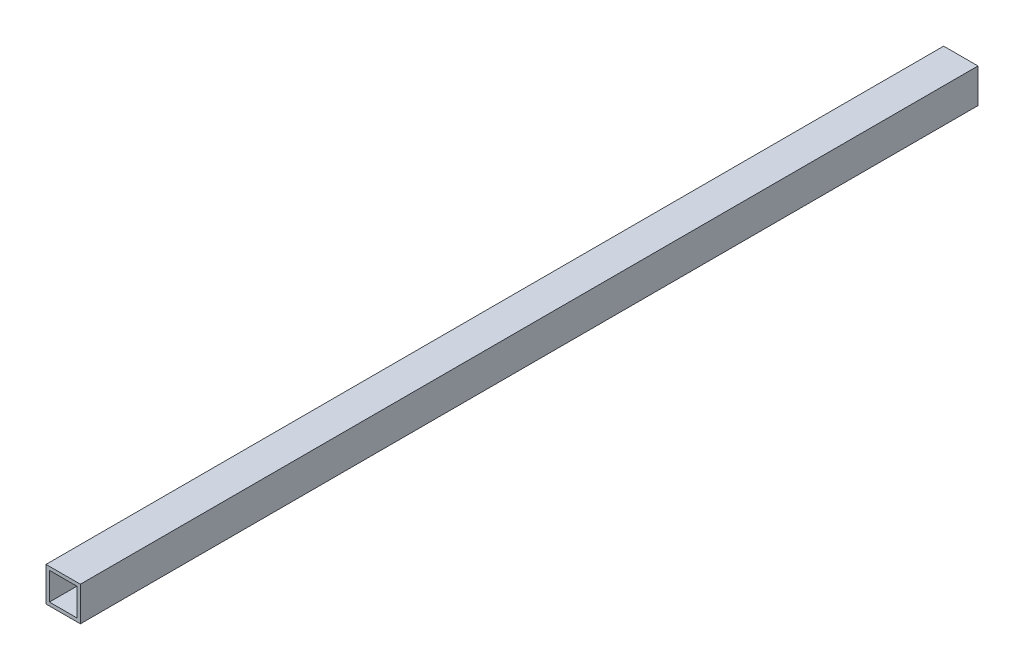
SolidWorks part; units mm, degrees
ref_plane "Front Plane" through (0, 0, 0) normal (0, 0, 1) x (1, 0, 0)
ref_plane "Top Plane" through (0, 0, 0) normal (0, 1, 0) x (1, 0, 0)
ref_plane "Right Plane" through (0, 0, 0) normal (1, 0, 0) x (0, 0, -1)
other "Configuration Table"
sketch "Sketch1" plane through (0, 0, 0) normal (0, 0, 1) x (1, 0, 0)
  line L0 (-16.1154, 15.8464) -> (13.8846, 15.8464)
  line L1 (13.8846, 15.8464) -> (13.8846, -14.1536)
  line L2 (13.8846, -14.1536) -> (-16.1154, -14.1536)
  line L3 (-16.1154, -14.1536) -> (-16.1154, 15.8464)
  line L4 (-13.1154, 12.8464) -> (10.8846, 12.8464)
  line L5 (10.8846, 12.8464) -> (10.8846, -11.1536)
  line L6 (10.8846, -11.1536) -> (-13.1154, -11.1536)
  line L7 (-13.1154, -11.1536) -> (-13.1154, 12.8464)
  dimension "D1" = 30
  dimension "D2" = 30
  dimension "D3" = 3
  dimension "D4" = 3
  dimension "D5" = 3
  dimension "D6" = 3
extrude "Boss-Extrude2" add sketch "Sketch1" along normal blind 784
